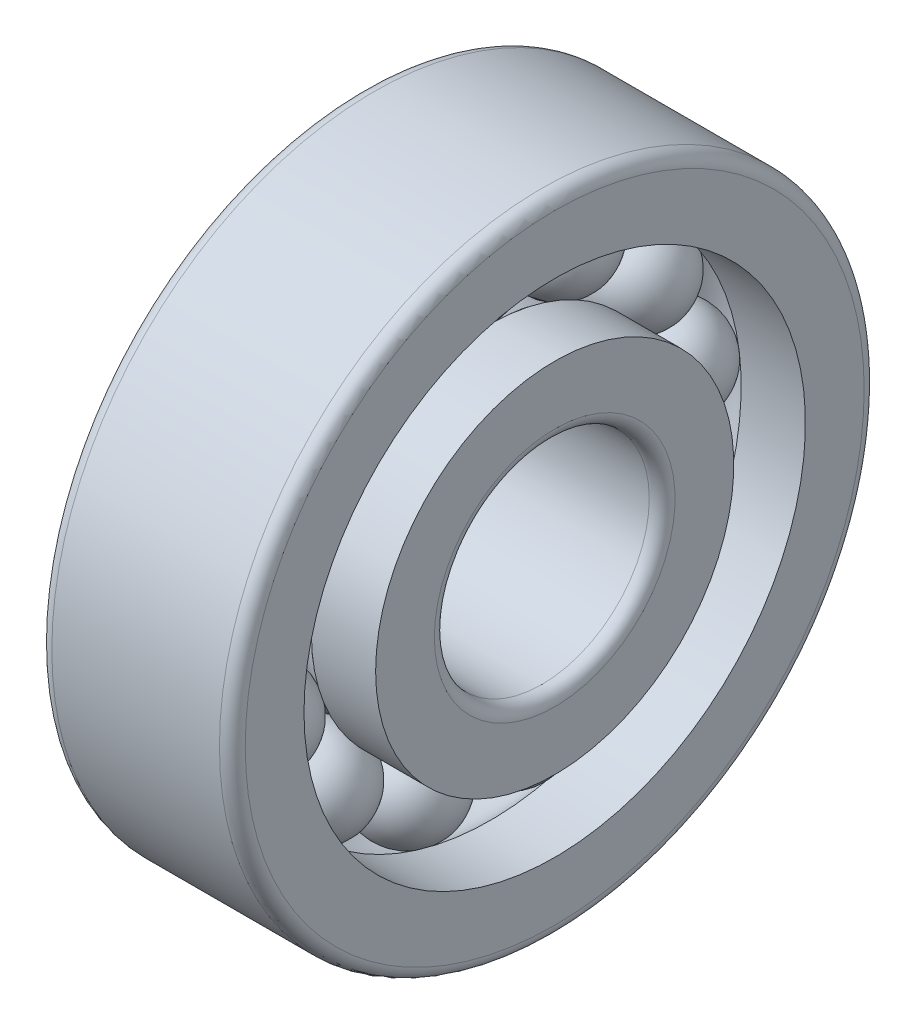
from build123d import *

# Parameters (mm, degrees)
PATTERN_CIRCULAR_5_COUNT = 13


with BuildPart() as part:
    # 草图2 → 旋转1 (revolve)
    with BuildSketch(Plane.XY, mode=Mode.PRIVATE) as revolve_1_sk:
        with BuildLine():
            Line((-4.2, 8.333333333), (-4.5, 8.333333333))
            Line((-4.5, 8.333333333), (-4.5, 7.733333333))
            Line((-4.5, 7.733333333), (-4.5, 5.6))
            ThreePointArc((-4.5, 5.6), (-4.324264069, 5.175735931), (-3.9, 5))
            Line((-3.9, 5), (3.9, 5))
            ThreePointArc((3.9, 5), (4.324264069, 5.175735931), (4.5, 5.6))
            Line((4.5, 5.6), (4.5, 7.733333333))
            Line((4.5, 7.733333333), (4.5, 8.333333333))
            Line((4.5, 8.333333333), (3.9, 8.333333333))
            Line((3.9, 8.333333333), (1.511529762, 8.333333333))
            ThreePointArc((1.511529762, 8.333333333), (0, 7.75), (-1.511529762, 8.333333333))
            Line((-1.511529762, 8.333333333), (-3, 8.333333333))
            Line((-3, 8.333333333), (-3, 7.733333333))
            Line((-3, 7.733333333), (-3.6, 7.733333333))
            Line((-3.6, 7.733333333), (-4.2, 8.333333333))
        make_face()
        with BuildLine():
            Line((-4.5, 11.666666667), (-4.2, 11.666666667))
            Line((-4.2, 11.666666667), (-3.6, 12.266666667))
            Line((-3.6, 12.266666667), (-3, 12.266666667))
            Line((-3, 12.266666667), (-3, 11.666666667))
            Line((-3, 11.666666667), (-1.511529762, 11.666666667))
            ThreePointArc((-1.511529762, 11.666666667), (0, 12.25), (1.511529762, 11.666666667))
            Line((1.511529762, 11.666666667), (4.5, 11.666666667))
            Line((4.5, 11.666666667), (4.5, 14.4))
            ThreePointArc((4.5, 14.4), (4.324264069, 14.824264069), (3.9, 15))
            Line((3.9, 15), (-3.9, 15))
            ThreePointArc((-3.9, 15), (-4.324264069, 14.824264069), (-4.5, 14.4))
            Line((-4.5, 14.4), (-4.5, 11.666666667))
        make_face()
    revolve(revolve_1_sk.sketch.rotate(Axis((-3.5, 0, 0), (1, 0, 0)), 90), axis=Axis((-3.5, 0, 0), (1, 0, 0)))


with BuildPart() as body_2:
    # 草图3 → 旋转2 (revolve)
    with BuildSketch(Plane.XY):
        with BuildLine():
            Line((-2.25, 10), (2.25, 10))
            ThreePointArc((2.25, 10), (0, 12.25), (-2.25, 10))
        make_face()
    revolve(axis=Axis((2.25, 10, 0), (1, 0, 0)))


with BuildPart() as body_3:
    # 草图4 → 旋转3 (revolve)
    with BuildSketch(Plane.XY, mode=Mode.PRIVATE) as revolve_3_sk:
        Polygon((-4.2, 11.666666667), (-4.2, 8.333333333), (-3.6, 7.733333333), (-3, 7.733333333), (-3, 8.333333333), (-3.6, 8.933333333), (-3.6, 11.066666667), (-3, 11.666666667), (-3, 12.266666667), (-3.6, 12.266666667), align=None)
    revolve(revolve_3_sk.sketch.rotate(Axis((-19.927092192, 0, 0), (1, 0, 0)), 90), axis=Axis((-19.927092192, 0, 0), (1, 0, 0)))


with BuildPart() as pattern_circular_5_1:
    # 阵列(圆周)5: pattern copy
    add(body_2.part.rotate(Axis((0, 0, 0), (1, 0, 0)), 1 * 360 / PATTERN_CIRCULAR_5_COUNT))


with BuildPart() as pattern_circular_5_2:
    # 阵列(圆周)5: pattern copy
    add(body_2.part.rotate(Axis((0, 0, 0), (1, 0, 0)), 2 * 360 / PATTERN_CIRCULAR_5_COUNT))


with BuildPart() as pattern_circular_5_3:
    # 阵列(圆周)5: pattern copy
    add(body_2.part.rotate(Axis((0, 0, 0), (1, 0, 0)), 3 * 360 / PATTERN_CIRCULAR_5_COUNT))


with BuildPart() as pattern_circular_5_4:
    # 阵列(圆周)5: pattern copy
    add(body_2.part.rotate(Axis((0, 0, 0), (1, 0, 0)), 4 * 360 / PATTERN_CIRCULAR_5_COUNT))


with BuildPart() as pattern_circular_5_5:
    # 阵列(圆周)5: pattern copy
    add(body_2.part.rotate(Axis((0, 0, 0), (1, 0, 0)), 5 * 360 / PATTERN_CIRCULAR_5_COUNT))


with BuildPart() as pattern_circular_5_6:
    # 阵列(圆周)5: pattern copy
    add(body_2.part.rotate(Axis((0, 0, 0), (1, 0, 0)), 6 * 360 / PATTERN_CIRCULAR_5_COUNT))


with BuildPart() as pattern_circular_5_7:
    # 阵列(圆周)5: pattern copy
    add(body_2.part.rotate(Axis((0, 0, 0), (1, 0, 0)), 7 * 360 / PATTERN_CIRCULAR_5_COUNT))


with BuildPart() as pattern_circular_5_8:
    # 阵列(圆周)5: pattern copy
    add(body_2.part.rotate(Axis((0, 0, 0), (1, 0, 0)), 8 * 360 / PATTERN_CIRCULAR_5_COUNT))


with BuildPart() as pattern_circular_5_9:
    # 阵列(圆周)5: pattern copy
    add(body_2.part.rotate(Axis((0, 0, 0), (1, 0, 0)), 9 * 360 / PATTERN_CIRCULAR_5_COUNT))


with BuildPart() as pattern_circular_5_10:
    # 阵列(圆周)5: pattern copy
    add(body_2.part.rotate(Axis((0, 0, 0), (1, 0, 0)), 10 * 360 / PATTERN_CIRCULAR_5_COUNT))


with BuildPart() as pattern_circular_5_11:
    # 阵列(圆周)5: pattern copy
    add(body_2.part.rotate(Axis((0, 0, 0), (1, 0, 0)), 11 * 360 / PATTERN_CIRCULAR_5_COUNT))


with BuildPart() as pattern_circular_5_12:
    # 阵列(圆周)5: pattern copy
    add(body_2.part.rotate(Axis((0, 0, 0), (1, 0, 0)), 12 * 360 / PATTERN_CIRCULAR_5_COUNT))


solid = Compound([part.part, body_2.part, body_3.part, pattern_circular_5_1.part, pattern_circular_5_2.part, pattern_circular_5_3.part, pattern_circular_5_4.part, pattern_circular_5_5.part, pattern_circular_5_6.part, pattern_circular_5_7.part, pattern_circular_5_8.part, pattern_circular_5_9.part, pattern_circular_5_10.part, pattern_circular_5_11.part, pattern_circular_5_12.part])
